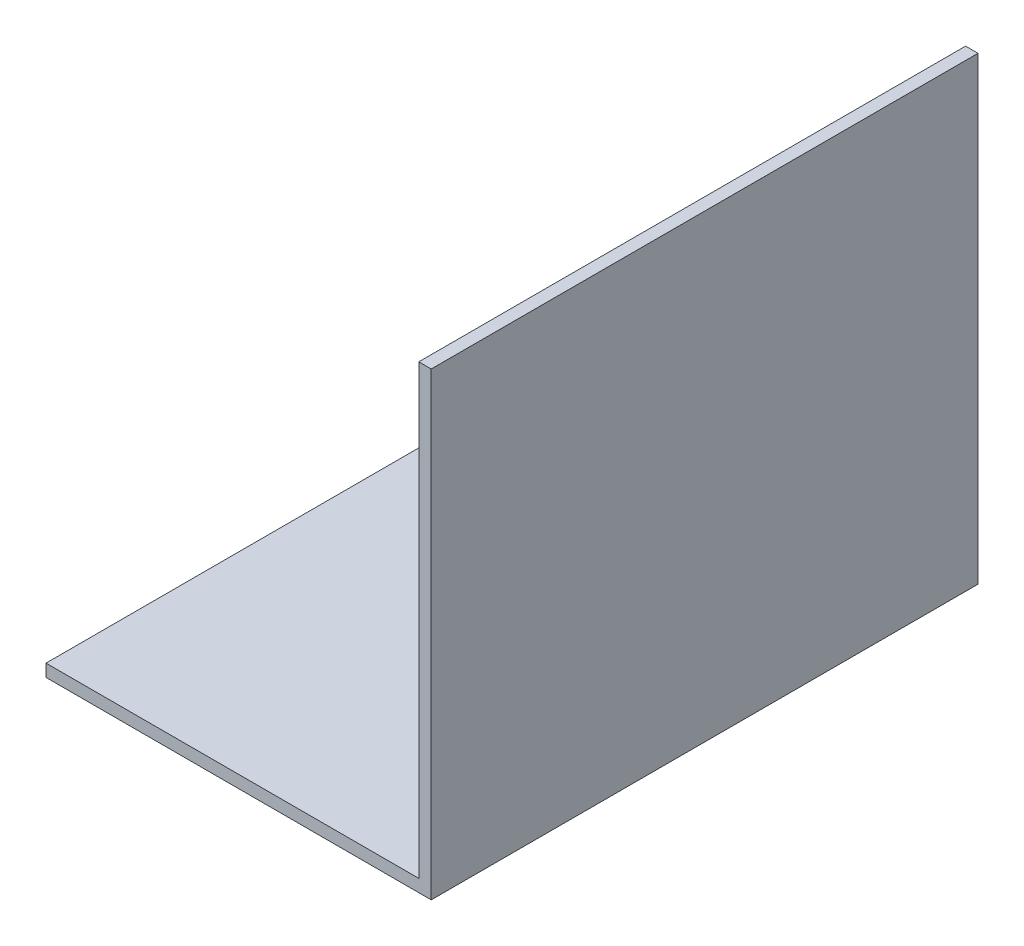
SolidWorks part; units mm, degrees
ref_plane "前视基准面" through (0, 0, 0) normal (0, 0, 1) x (1, 0, 0)
ref_plane "上视基准面" through (0, 0, 0) normal (0, 1, 0) x (1, 0, 0)
ref_plane "右视基准面" through (0, 0, 0) normal (1, 0, 0) x (0, 0, -1)
other "Configuration Table"
sketch "草图1" plane through (0, 0, 0) normal (0, 0, 1) x (1, 0, 0)
  line L0 (-155, 0) -> (0, 0)
  line L1 (0, 0) -> (0, 185)
  line L2 (0, 185) -> (-5, 185)
  line L3 (-5, 185) -> (-5, 5)
  line L4 (-5, 5) -> (-155, 5)
  line L5 (-155, 5) -> (-155, 0)
  point P0 (0, 0)
  dimension "D1" = 5
  dimension "D2" = 155
  dimension "D3" = 180
  dimension "D4" = 185
extrude "凸台-拉伸1" add sketch "草图1" against normal mid plane 220
